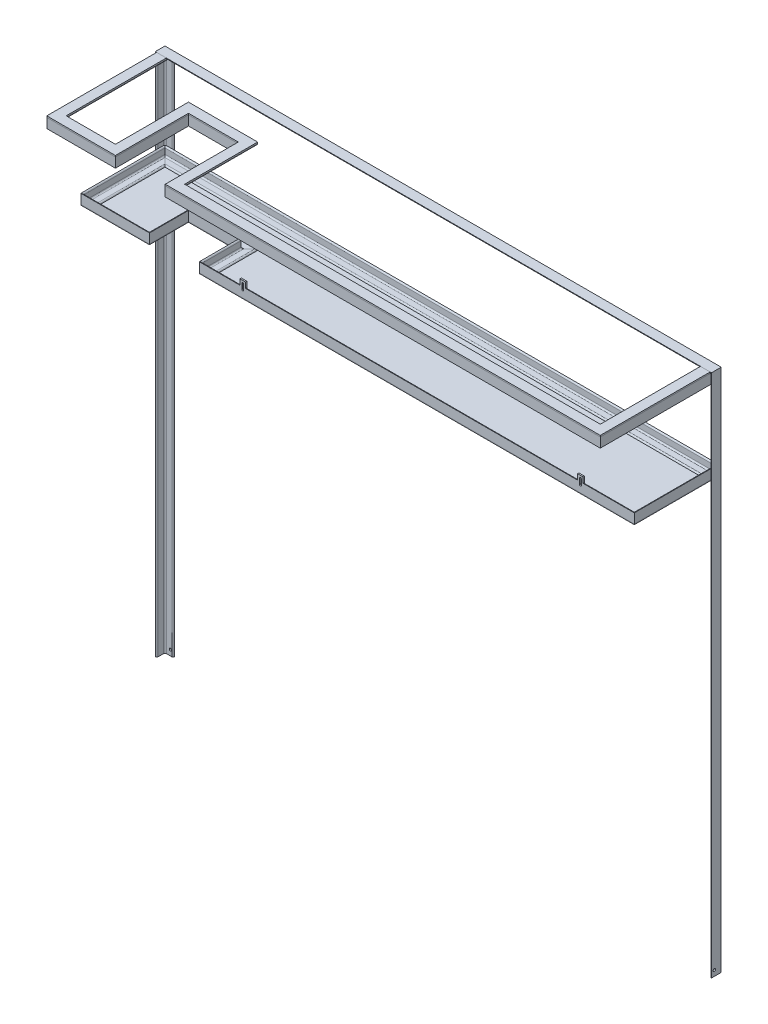
SolidWorks part; units mm, degrees
ref_plane "前视基准面" through (0, 0, 0) normal (0, 0, 1) x (1, 0, 0)
ref_plane "上视基准面" through (0, 0, 0) normal (0, 1, 0) x (1, 0, 0)
ref_plane "右视基准面" through (0, 0, 0) normal (1, 0, 0) x (0, 0, -1)
sketch "草图1" plane through (0, 0, 0) normal (0, 0, 1) x (1, 0, 0)
  line L0 (0, 0) -> (2010, 0)
  line L1 (0, 0) -> (0, -1894)
  line L2 (2010, 0) -> (2010, -1894)
  dimension "D1" = 2010
  dimension "D2" = 1894
  dimension "D3" = 1894
other "结构构件1"
ref_plane "基准面1" through (0, 0, 0) normal (1, 0, 0) x (0, 0, 1)
sketch "Sketch1" plane through (0, 0, 0) normal (1, 0, 0) x (0, 0, 1)
  line L0 (0, 0) -> (0, 35)
  line L1 (0, 17.5) -> (5, 17.5) construction
  line L2 (5, 30) -> (5, 10)
  line L3 (10, 5) -> (30, 5)
  line L4 (17.5, 5) -> (17.5, 0) construction
  line L5 (35, 0) -> (0, 0)
  arc A0 (35, 0) -> (30, 5) centre (30, 0) ccw
  arc A1 (0, 35) -> (5, 30) centre (0, 30) cw
  arc A2 (10, 5) -> (5, 10) centre (10, 10) cw
  point P10 (17.5, 0)
  point P14 (0, 17.5)
  point P15 (5, 17.5)
  point P16 (17.5, 5)
  point P17 (5, 35)
  point P18 (35, 5)
  point P21 (0, 0)
  dimension "D2" = 5
  dimension "D3" = 35
  dimension "Radius_1" = 5
  dimension "D1" = 5
sketch "草图3" plane through (0, -5, 0) normal (0, -1, 0) x (1, 0, 0)
  line L0 (5, 5) -> (5, 432)
  line L1 (2005, 5) -> (2005, 432)
  line L2 (2005, 432) -> (433, 432)
  line L3 (2005, 30) -> (2005, 10) construction
  line L4 (2000, 5) -> (1980, 5) construction
  line L5 (5, 30) -> (5, 10) construction
  line L6 (5, 10) -> (5, 30) construction
  line L7 (253, 432) -> (253, 168)
  line L8 (253, 168) -> (433, 168)
  line L9 (433, 168) -> (433, 432)
  line L10 (253, 432) -> (5, 432)
  dimension "D1" = 248
  dimension "D2" = 180
  dimension "D3" = 427
  dimension "D4" = 264
other "结构构件2"
ref_plane "基准面2" through (5, -5, 5) normal (0, 0, 1) x (0, -1, 0)
sketch "Sketch11" plane through (5, -5, 5) normal (0, 0, 1) x (0, -1, 0)
  line L0 (0, 0) -> (0, 35)
  line L1 (0, 17.5) -> (5, 17.5) construction
  line L2 (5, 30) -> (5, 10)
  line L3 (10, 5) -> (30, 5)
  line L4 (17.5, 5) -> (17.5, 0) construction
  line L5 (35, 0) -> (0, 0)
  arc A0 (35, 0) -> (30, 5) centre (30, 0) ccw
  arc A1 (0, 35) -> (5, 30) centre (0, 30) cw
  arc A2 (10, 5) -> (5, 10) centre (10, 10) cw
  point P10 (17.5, 0)
  point P14 (0, 17.5)
  point P15 (5, 17.5)
  point P16 (17.5, 5)
  point P17 (5, 35)
  point P18 (35, 5)
  point P21 (0, 0)
  dimension "D2" = 5
  dimension "D3" = 35
  dimension "Radius_1" = 5
  dimension "D1" = 5
ref_plane "基准面3" through (0, -339, 0) normal (0, 1, 0) x (-1, 0, 0)
sketch "草图5" plane through (0, -339, 0) normal (0, 1, 0) x (-1, 0, 0)
  line L0 (-2005, 5) -> (-2005, 309)
  line L1 (-2005, 5) -> (-2005, 432) construction
  line L2 (-2005, 309) -> (-433, 309)
  line L3 (-5, 432) -> (-5, 5) construction
  line L4 (-5, 309) -> (-5, 5)
  line L5 (-433, 309) -> (-433, 168)
  line L6 (-433, 168) -> (-253, 168)
  line L7 (-253, 168) -> (-253, 309)
  line L8 (-2010, 35) -> (0, 35) construction
  line L9 (-253, 309) -> (-5, 309)
  line L13 (-2005, 5) -> (-5, 5)
  dimension "D1" = 304
  dimension "D2" = 141
  dimension "D3" = 248
  dimension "D4" = 180
other "结构构件3"
ref_plane "基准面4" through (2005, -339, 5) normal (0, 0, 1) x (0, 1, 0)
sketch "Sketch12" plane through (2005, -339, 5) normal (0, 0, 1) x (0, 1, 0)
  line L0 (0, 0) -> (0, 35)
  line L1 (0, 17.5) -> (5, 17.5) construction
  line L2 (5, 30) -> (5, 10)
  line L3 (10, 5) -> (30, 5)
  line L4 (17.5, 5) -> (17.5, 0) construction
  line L5 (35, 0) -> (0, 0)
  arc A0 (35, 0) -> (30, 5) centre (30, 0) ccw
  arc A1 (0, 35) -> (5, 30) centre (0, 30) cw
  arc A2 (10, 5) -> (5, 10) centre (10, 10) cw
  point P10 (17.5, 0)
  point P14 (0, 17.5)
  point P15 (5, 17.5)
  point P16 (17.5, 5)
  point P17 (5, 35)
  point P18 (35, 5)
  point P21 (0, 0)
  dimension "D2" = 5
  dimension "D3" = 35
  dimension "Radius_1" = 5
  dimension "D1" = 5
sketch "草图8" plane through (0, 0, 5) normal (0, 0, 1) x (1, 0, 0)
  line L0 (35, -35) -> (35, -1894) construction
  line L1 (10, -1894) -> (30, -1894) construction
  line L2 (1219, -339) -> (1219, -2038.6334) construction
  line L3 (433, -339) -> (2005, -339) construction
  circle A0 centre (25, -1874) radius 4.5
  circle A1 centre (2413, -1874) radius 4.5
  dimension "D1" = 9
  dimension "D2" = 10
  dimension "D3" = 20
extrude "切除-拉伸1" cut sketch "草图8" against normal blind 10
sketch "草图9" plane through (0, 0, 0) normal (-1, 0, 0) x (0, 0, 1)
  line L0 (35, 0) -> (35, -1894) construction
  line L1 (0, -1894) -> (35, -1894) construction
  circle A0 centre (25, -1874) radius 4.5
  dimension "D1" = 9
  dimension "D2" = 10
  dimension "D3" = 20
extrude "切除-拉伸2" cut sketch "草图9" against normal blind 2440 from offset 50 offset against normal yes
sketch "草图11" plane through (0, -5, 0) normal (0, 1, 0) x (1, 0, 0)
  line L41 (2005, -5) -> (2005, -432)
  line L42 (2005, -432) -> (433, -432)
  line L43 (433, -432) -> (433, -168)
  line L44 (433, -168) -> (253, -168)
  line L45 (253, -168) -> (253, -432)
  line L46 (253, -432) -> (5, -432)
  line L47 (5, -432) -> (5, -5)
  line L48 (2005, -35) -> (2005, -432)
  line L49 (2005, -432) -> (433, -432)
  line L50 (433, -432) -> (433, -168)
  line L51 (433, -168) -> (253, -168)
  line L52 (253, -168) -> (253, -432)
  line L53 (253, -432) -> (5, -432)
  line L54 (5, -432) -> (5, -35)
  line L76 (5, -35) -> (40, -35)
  line L77 (2010, -35) -> (0, -35) construction
  line L78 (1970, -35) -> (2005, -35)
  line L83 (40, -397) -> (40, -5)
  line L84 (218, -397) -> (40, -397)
  line L85 (218, -133) -> (218, -397)
  line L86 (468, -133) -> (218, -133)
  line L87 (468, -397) -> (468, -133)
  line L88 (1970, -397) -> (468, -397)
  line L89 (1970, -5) -> (1970, -397)
  line L90 (40, -397) -> (40, -35)
  line L91 (218, -397) -> (40, -397)
  line L92 (218, -133) -> (218, -397)
  line L93 (468, -133) -> (218, -133)
  line L94 (468, -397) -> (468, -133)
  line L95 (1970, -397) -> (468, -397)
  line L96 (1970, -35) -> (1970, -397)
  dimension "D1" = 0
  dimension "D2" = 0
extrude "凸台-拉伸1" add sketch "草图11" along normal blind 5 separate body
sketch "草图13" plane through (0, -339, 0) normal (0, -1, 0) x (1, 0, 0)
  line L0 (5, 309) -> (5, 5)
  line L1 (5, 432) -> (5, 5) construction
  line L2 (2005, 5) -> (5, 5) construction
  line L3 (5, 5) -> (2005, 5)
  line L4 (1970, 40) -> (2005, 5) construction
  line L5 (2005, 5) -> (1970, 40) construction
  line L6 (2005, 5) -> (2005, 309)
  line L7 (2005, 309) -> (433, 309)
  line L8 (433, 309) -> (433, 168)
  line L9 (433, 168) -> (253, 168)
  line L10 (253, 168) -> (253, 309)
  line L11 (253, 309) -> (5, 309)
extrude "凸台-拉伸2" add sketch "草图13" along normal blind 2 separate body
sketch "草图14" plane through (0, 0, 309) normal (0, 0, 1) x (1, 0, 0)
  line L1 (580, -314) -> (600, -314)
  line L2 (580, -314) -> (580, -284)
  line L3 (580, -284) -> (600, -284)
  line L4 (600, -314) -> (600, -284)
  line L5 (433, -304) -> (2005, -304) construction
  line L6 (590, -284) -> (590, -365.4728) construction
  line L7 (2010, -1894) -> (2010, 0) construction
  line L8 (1810, -284) -> (1810, -382.8664) construction
  line L9 (1800, -284) -> (1820, -284)
  line L10 (1800, -284) -> (1800, -314)
  line L11 (1800, -314) -> (1820, -314)
  line L12 (1820, -284) -> (1820, -314)
  dimension "D1" = 10
  dimension "D2" = 30
  dimension "D3" = 20
  dimension "D4" = 1420
  dimension "D5" = 20
  dimension "D6" = 30
  dimension "D7" = 10
  dimension "D8" = 200
extrude "凸台-拉伸3" add sketch "草图14" against normal blind 5
sketch "草图15" plane through (0, 0, 304) normal (0, 0, -1) x (-1, 0, 0)
  line L0 (-1810, -284) -> (-1810, -357.4789) construction
  line L1 (-1820, -284) -> (-1800, -284) construction
  line L2 (-1833.5583, -294) -> (-1769.7688, -294) construction
  line L3 (-590, -284) -> (-590, -363.3833) construction
  line L4 (-600, -284) -> (-580, -284) construction
  line L5 (-510.9711, -294) -> (-463.7863, -294) construction
  line L6 (-1813.5, -294) -> (-1813.5, -314)
  line L7 (-1806.5, -294) -> (-1806.5, -314)
  line L8 (-593.5, -294) -> (-593.5, -314)
  line L9 (-586.5, -294) -> (-586.5, -314)
  arc A0 (-1806.5, -294) -> (-1813.5, -294) centre (-1810, -294) ccw
  arc A1 (-586.5, -294) -> (-593.5, -294) centre (-590, -294) ccw
  arc A2 (-1813.5, -314) -> (-1806.5, -314) centre (-1810, -314) ccw
  arc A3 (-593.5, -314) -> (-586.5, -314) centre (-590, -314) ccw
  dimension "D2" = 7
  dimension "D3" = 7
  dimension "D4" = 7
  dimension "D5" = 20
  dimension "D7" = 7
  dimension "D8" = 20
  dimension "D1" = 10
  dimension "D6" = 7
  dimension "D9" = 7
extrude "切除-拉伸3" cut sketch "草图15" against normal blind 5
